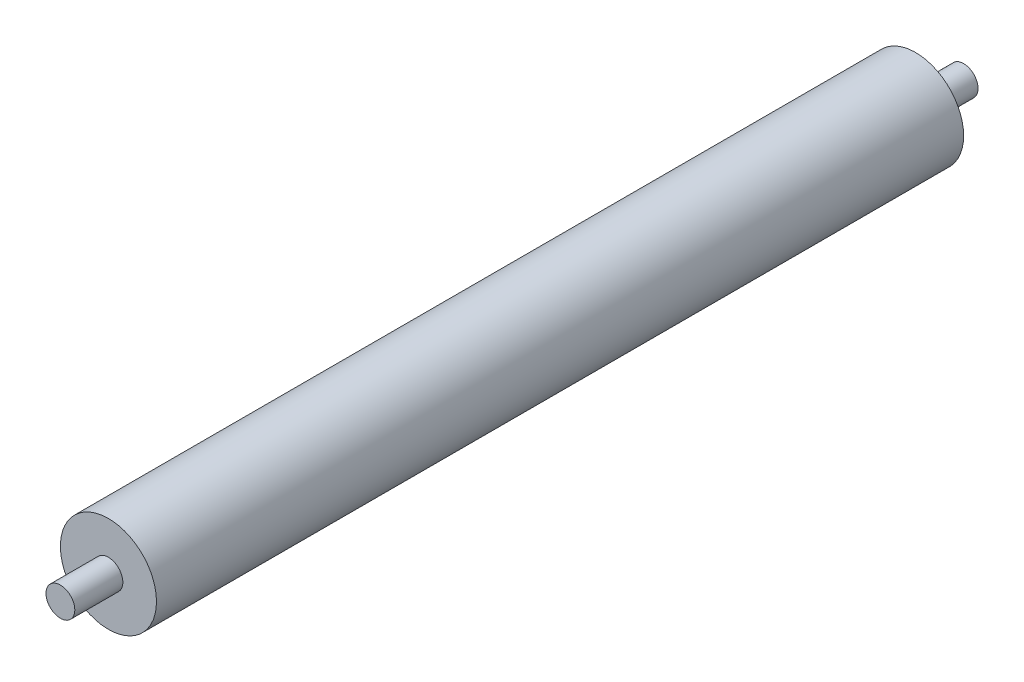
SolidWorks part; units mm, degrees
ref_plane "前视基准面" through (0, 0, 0) normal (0, 0, 1) x (1, 0, 0)
ref_plane "上视基准面" through (0, 0, 0) normal (0, 1, 0) x (1, 0, 0)
ref_plane "右视基准面" through (0, 0, 0) normal (1, 0, 0) x (0, 0, -1)
sketch "草图1" plane through (0, 0, 0) normal (0, 0, 1) x (1, 0, 0)
  circle A0 centre (0, 0) radius 25
  dimension "D1" = 50
extrude "凸台-拉伸1" add sketch "草图1" along normal blind 420
sketch "草图2" plane through (0, 0, 420) normal (0, 0, 1) x (1, 0, 0)
  circle A0 centre (0, 0) radius 7.5
  dimension "D1" = 15
extrude "凸台-拉伸2" add sketch "草图2" along normal blind 25
sketch "草图3" plane through (0, 0, 0) normal (0, 0, -1) x (-1, 0, 0)
  circle A0 centre (0, 0) radius 7.5
  dimension "D1" = 15
extrude "凸台-拉伸3" add sketch "草图3" along normal blind 25
